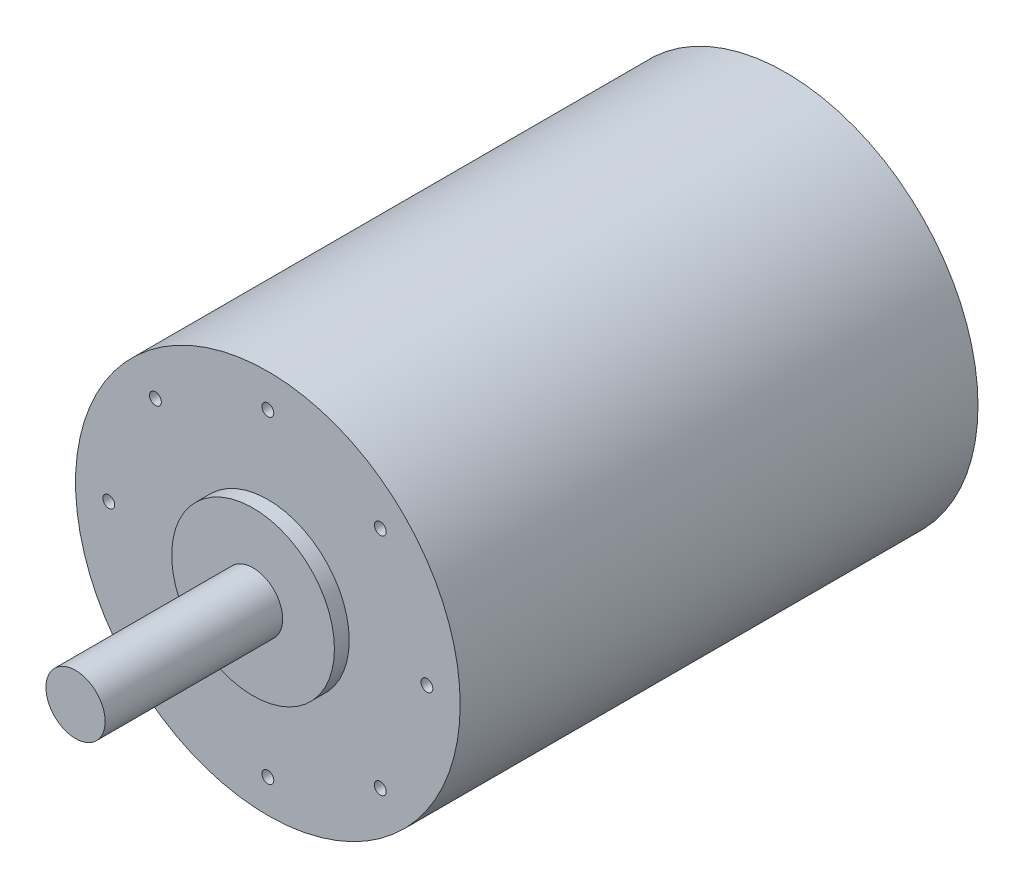
from build123d import *

# Parameters (mm, degrees)
SKETCH_1_R             = 26
EXTRUDE_1_DEPTH        = 70
SKETCH_2_R             = 11
EXTRUDE_2_DEPTH        = 2
SKETCH_3_R             = 4
EXTRUDE_3_DEPTH        = 24
HOLE_WIZARD_M2_1_D     = 1.6
HOLE_WIZARD_M2_1_DEPTH = 5.2
HOLE_WIZARD_M2_1_TIP   = 0.480688495


with BuildPart() as part:
    # 草图1 → 凸台-拉伸1 (new body)
    with BuildSketch(Plane.XY):
        Circle(SKETCH_1_R)
    extrude(amount=EXTRUDE_1_DEPTH)

    # 草图2 → 凸台-拉伸2 (add)
    with BuildSketch(Plane.XY.offset(70)):
        Circle(SKETCH_2_R)
    extrude(amount=EXTRUDE_2_DEPTH)

    # 草图3 → 凸台-拉伸3 (add)
    with BuildSketch(Plane.XY.offset(72)):
        Circle(SKETCH_3_R)
    extrude(amount=EXTRUDE_3_DEPTH)

    # M2 螺纹孔1
    with Locations(Plane.XY.offset(70)):
        with Locations((0, 21.5), (15.202795796, 15.202795796), (21.5, 0), (15.202795796, -15.202795796), (0, -21.5), (-15.202795796, -15.202795796), (-21.5, 0), (-15.202795796, 15.202795796)):
            Hole(HOLE_WIZARD_M2_1_D / 2, depth=HOLE_WIZARD_M2_1_DEPTH)
            with Locations((0, 0, -(HOLE_WIZARD_M2_1_DEPTH + HOLE_WIZARD_M2_1_TIP / 2))):  # 118° drill point
                Cone(0, HOLE_WIZARD_M2_1_D / 2, HOLE_WIZARD_M2_1_TIP, mode=Mode.SUBTRACT)


solid = part.part
